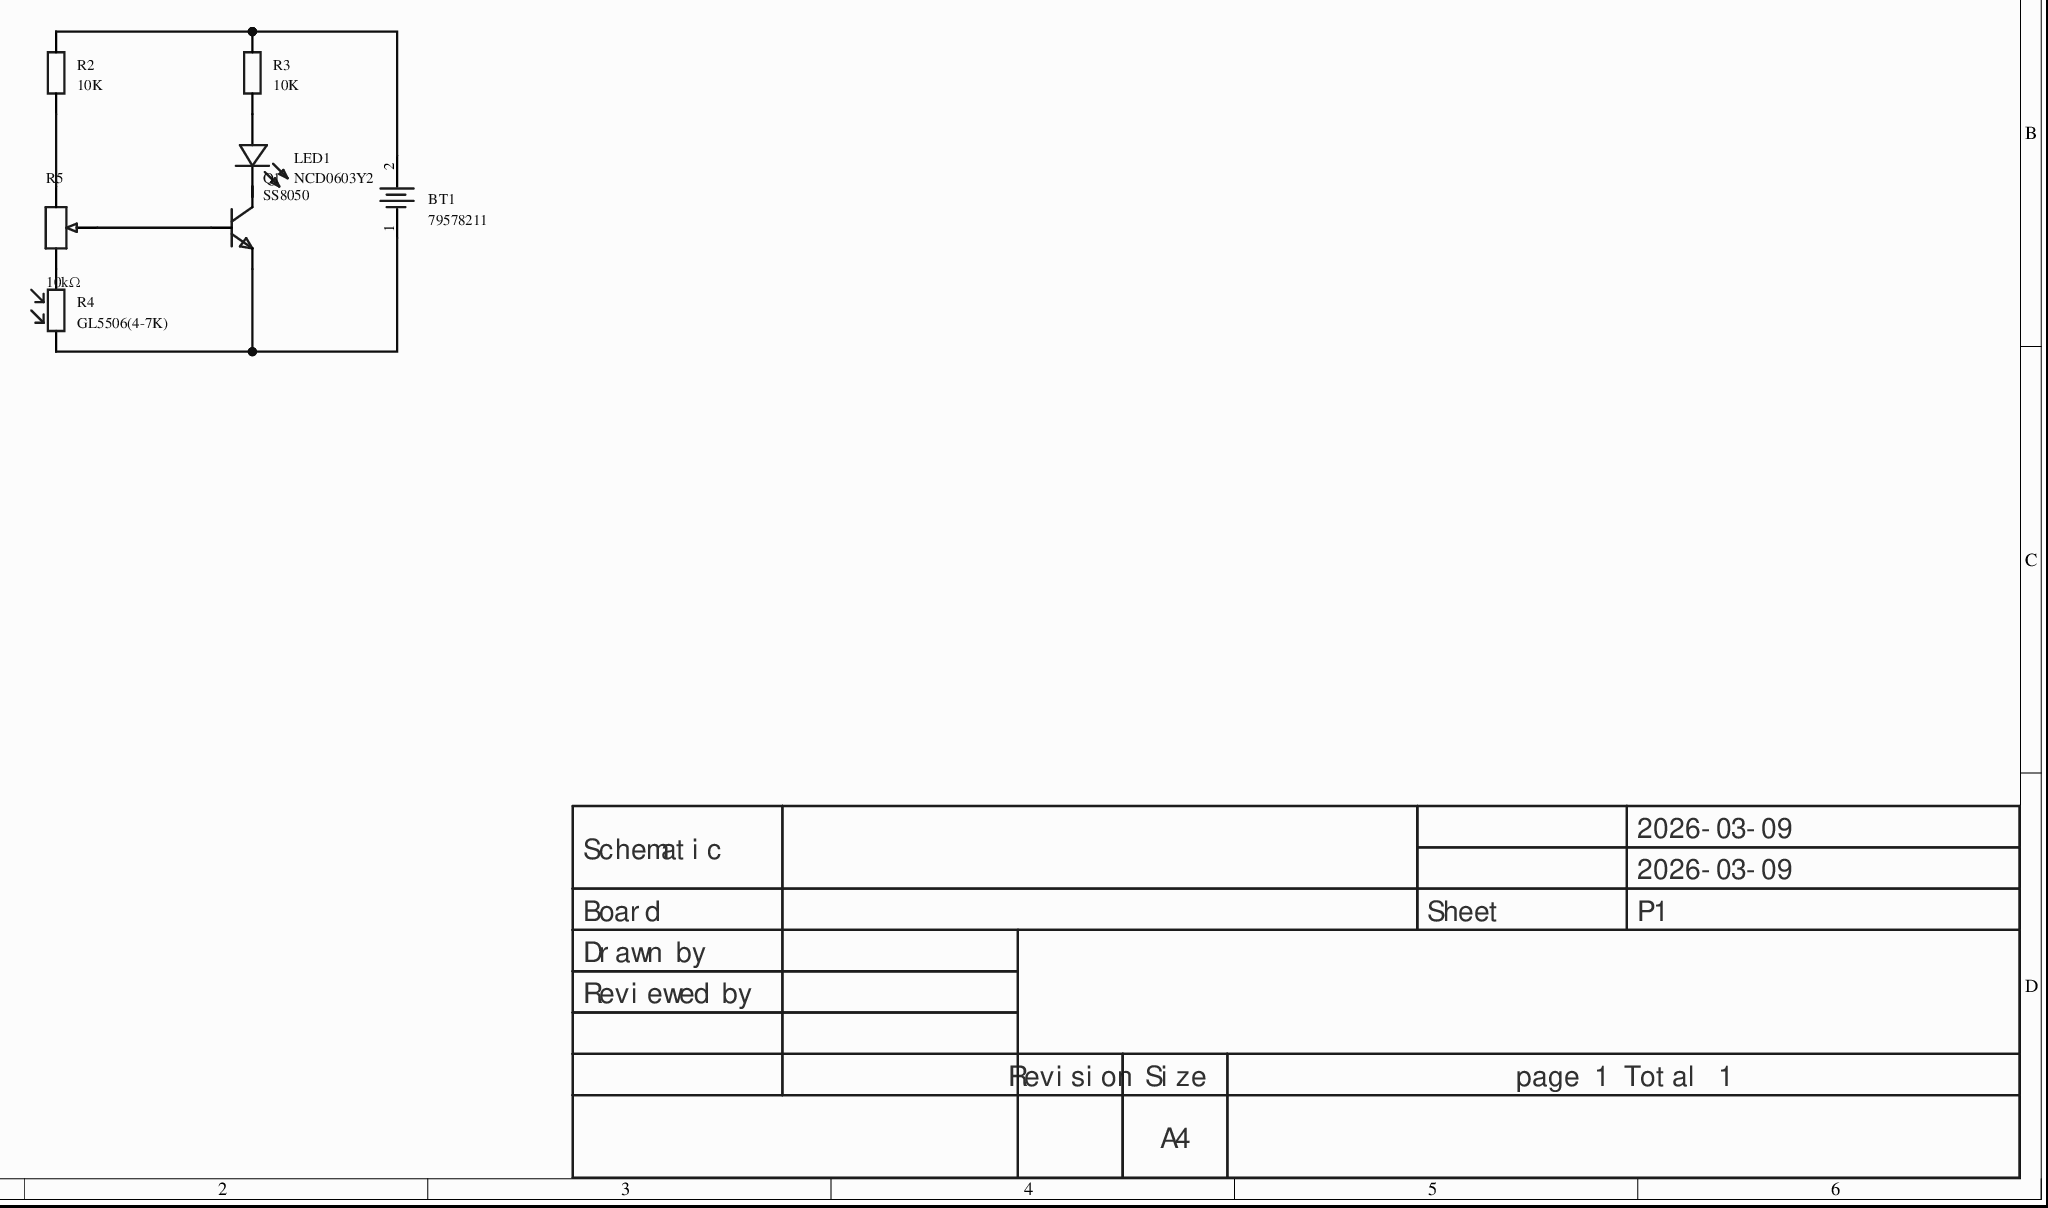
[diagram p0: MISC51971-3.schdoc]
# Altium project MISC51971-2.PrjPcb
1 sheet, 7 parts. Net scope: global (net labels, ports and power ports of the same name join across sheets).
Board file: MISC51971.pcbdoc

## Sheet MISC51971-3.schdoc
size 297 x 209 mm; Version: V1.0; @Project Name: MISC51971; @Update Date: 2026-03-09; @Create Date: 2026-03-09; @Board Name: MISC51971; @Create Time: 03:12:08; @Page Count: 1; @Page No: 1; @Schematic Name: MISC51971; @Update Time: 03:12:08; Size: A4

### Parts
BT1  79578211  [BAT-TH_79578211]
LED1  NCD0603Y2  [LED0603-RD]
Q1  SS8050  [SOT-23-3_L2.9-W1.3-P1.90-LS2.4-BR]
R2  10K  [R0603]
R3  10K  [R0603]
R4  GL5506(4-7K)  [RES-TH_L5.1-W4.3-P3.00-D0.5]
R5  10kΩ  [RES-ADJ-TH_RDC1022A05]

### Nets
NetBT1_1: BT1.1(-) Q1.2(E) R4.2
NetBT1_2: BT1.2(+) R2.2 R3.2
NetLED1_1: LED1.1(K) Q1.3(C)
NetLED1_2: LED1.2(A) R3.1
NetQ1_1: Q1.1(B) R5.2
NetR2_1: R2.1 R5.3
NetR4_1: R4.1 R5.1

### Notes on the sheet
- 2026-03-09
- Schematic
- Board
- Sheet
- P1
- Drawn by
- Reviewed by
- Revision
- Size
- A4
- page 1 Total 1

### Library data of the parts
BT1 = 79578211: 特性：基础材料:PBT。基础阻燃等级:UL94 V 0。基础颜色:黑色。接触材料:磷青铜。接触镀层:镍(Ni)。额定电流:0.5 A。耐受电压:12 V(DC)。接触电阻:最大30 mΩ。绝缘电阻:最小100 MΩ。RoHS认证:符合[2011/65/EU&2015/863]。REACH认证:符合或声明[(EC)1907/2006]。无卤:符合[IEC 61249 2 21]。无卤:符合[JEDEC JS709B]。工作温度:-25至+85 °C。储存条件(原包装):温度&lt; 40 °C;相对湿度&l; Manufacturer: Wurth(伍尔特); AddInBom: yes; ModelId: 711ad6e3f27f4ce9b3480f737ec158fb0819f05c4eef4c71ace90d822a990e87; ModelTransform: 1154.347,1053.10061,0,0,0,0,141.732,0,-125.984; Symbol: 79578211; Device: 79578211; LCSC Part Name: 直流电源插孔，SMT，卧式，带定位销，O2.00mm; SupplierPart: C5544866; ManufacturerPart: 79578211; Supplier Footprint: -; JLCPCB Part Class: Extended Part; Datasheet: https://www.we-online.com/components/products/datasheet/79578211.pdf; Supplier: LCSC; ConvertToPcb: yes; FootprintName: BAT-TH_79578211; ModelName: BAT-TH_79578211
LED1 = NCD0603Y2: Emitted color: yellow; forward voltage (VF): 1.6V~2.6V; power: 65mW; forward current: 20mA; dominant wavelength: 586nm~595nm; lens color: colorless transparent lens; luminous intensity: 100mcd~220mcd; viewing angle: 130°; operating temperature: -30℃~+85℃;; Manufacturer: 国星光电; Symbol: FC-1608YXK-585F08; AddInBom: yes; ModelId: 1f0d29a91be547639d425604e9b96ebb0819f05c4eef4c71ace90d822a990e87; ModelTransform: 63.7794,32.283,0,0,0,0,0,0,0; Device: NCD0603Y2; LCSC Part Name: NCD0603Y2; SupplierPart: C89811; ManufacturerPart: NCD0603Y2; Supplier Footprint: 0603; JLCPCB Part Class: Extended Part; Datasheet: https://atta.szlcsc.com/upload/public/pdf/source/20200820/C89811_7FE84B429B6BCA3E113B125EE1452576.pdf; Supplier: LCSC; ConvertToPcb: yes; FootprintName: LED0603-RD; ModelName: LED0603-RD; Emitted Color: Yellow; Forward Voltage (VF): 1.6V~2.6V; Power Dissipation: 65mW; Forward Current: 20mA; Dominant Wavelength: 586nm~595nm; Lens Color: Colorless transparent lens; Luminous Intensity: 100mcd~220mcd; Viewing Angle: 130°; Operating Temperature: -30℃~+85℃
Q1 = SS8050_C7420370: Transistor type: NPN; collector current (Ic): 1.5A; collector-emitter breakdown voltage (Vceo): 25V; power dissipation (Pd): 300mW; DC current gain (hFE): 120@100mA,1.0V;; Manufacturer: R+O(宏嘉诚); AddInBom: yes; ModelId: c62791f0466c4ae2a892c056b845b0ca0819f05c4eef4c71ace90d822a990e87; ModelName: SOT-23-3P_L2.9-W1.3-H1.0-LS2.4-P0.95; ModelTransform: 98.425,114.173,0,180,0,0,0.0005,-0.0005,0; Transition frequency(fT): 100MHz; Current - Collector Cutoff: 100nA; Vce Saturation(VCE(sat)): 500mV; Emitter-Base Voltage(Vebo): 5V; Symbol: SS8050_C7420370; Device: SS8050_C7420370; LCSC Part Name: H档 200-350 NPN 电流:1.5A 电压:25V; SupplierPart: C7420370; ManufacturerPart: SS8050; Supplier Footprint: SOT-23; JLCPCB Part Class: Extended Part; Datasheet: https://item.szlcsc.com/datasheet/SS8050/8397192.html; Supplier: LCSC; ConvertToPcb: yes; FootprintName: SOT-23-3_L2.9-W1.3-P1.90-LS2.4-BR; type: NPN; Current - Collector(Ic): 1.5A; Collector - Emitter Voltage VCEO: 25V; Pd - Power Dissipation: 300mW; DC Current Gain: 120@100mA,1.0V; Operating Temperature: -55℃~+150℃
R2 R3 = Res_0603: Symbol: Resistor; ConvertToPcb: yes; ModelId: fc143cca1e79419f9cd78b61e9279f080819f05c4eef4c71ace90d822a990e87; ModelTransform: 31.8897,63.7794,0,90,0,0,0,0,0; Device: Res_0603; AddInBom: yes; Supplier Footprint: 0603; FootprintName: R0603; ModelName: R0603; Value: 10K
R4 = GL5506（4-7K）: Dark resistance: 500kΩ; light resistance @10Lux: 4kΩ~7kΩ; spectral peak (wavelength): 540nm;; Manufacturer: JCHL(晶创和立); AddInBom: yes; ModelId: 5d124d9955ea497c88b5d664bd1bf7b70819f05c4eef4c71ace90d822a990e87; ModelName: RES-TH_L5.1-W4.3-H2.1-P3.00-D0.5; ModelTransform: 200.787,169.291,0,0,0,0,0,0,-196.85; Voltage - Max: 150V; Rise Time: 30ms; γ Value: 0.5; Symbol: GL5506(4-7K); Device: GL5506(4-7K); LCSC Part Name: 电位器; SupplierPart: C11299; ManufacturerPart: GL5506（4-7K）; Supplier Footprint: 插件,P=3mm; JLCPCB Part Class: Extended Part; Datasheet: https://item.szlcsc.com/datasheet/GL5506%25EF%25BC%25884-7K%25EF%25BC%2589/11852.html; Supplier: LCSC; ConvertToPcb: yes; FootprintName: RES-TH_L5.1-W4.3-P3.00-D0.5; Dark Resistance: 500kΩ; Cell Resistance @ Illuminance: 4kΩ~7kΩ; Wavelength - Peak: 540nm; Fall Time: 30ms; Operating Temperature: -30℃~+70℃
R5 = RDC1022A05: Resistance: 10kΩ; tolerance: ±30%; power: -;; Manufacturer: ALPSALPINE(阿尔卑斯阿尔派); AddInBom: yes; ModelId: 6188e05200ce4e918c561a765f38371f0819f05c4eef4c71ace90d822a990e87; ModelTransform: 1240.155,431.102,0,0,0,0,-495.591,81.378,-137.795; Symbol: RDC1022A05; Device: RDC1022A05; LCSC Part Name: 10kΩ ±30%; SupplierPart: C202389; ManufacturerPart: RDC1022A05; Supplier Footprint: 插件; JLCPCB Part Class: Extended Part; Datasheet: https://atta.szlcsc.com/upload/public/pdf/source/20180403/C202389_1B1795B6045599E7FBF27F2153BF043E.pdf; Supplier: LCSC; ConvertToPcb: yes; FootprintName: RES-ADJ-TH_RDC1022A05; ModelName: RES-ADJ-TH_RDC1022A05; Value: 10kΩ; Tolerance: ±30%; Rated Voltage: -; Power(Watts): -; Turns: -